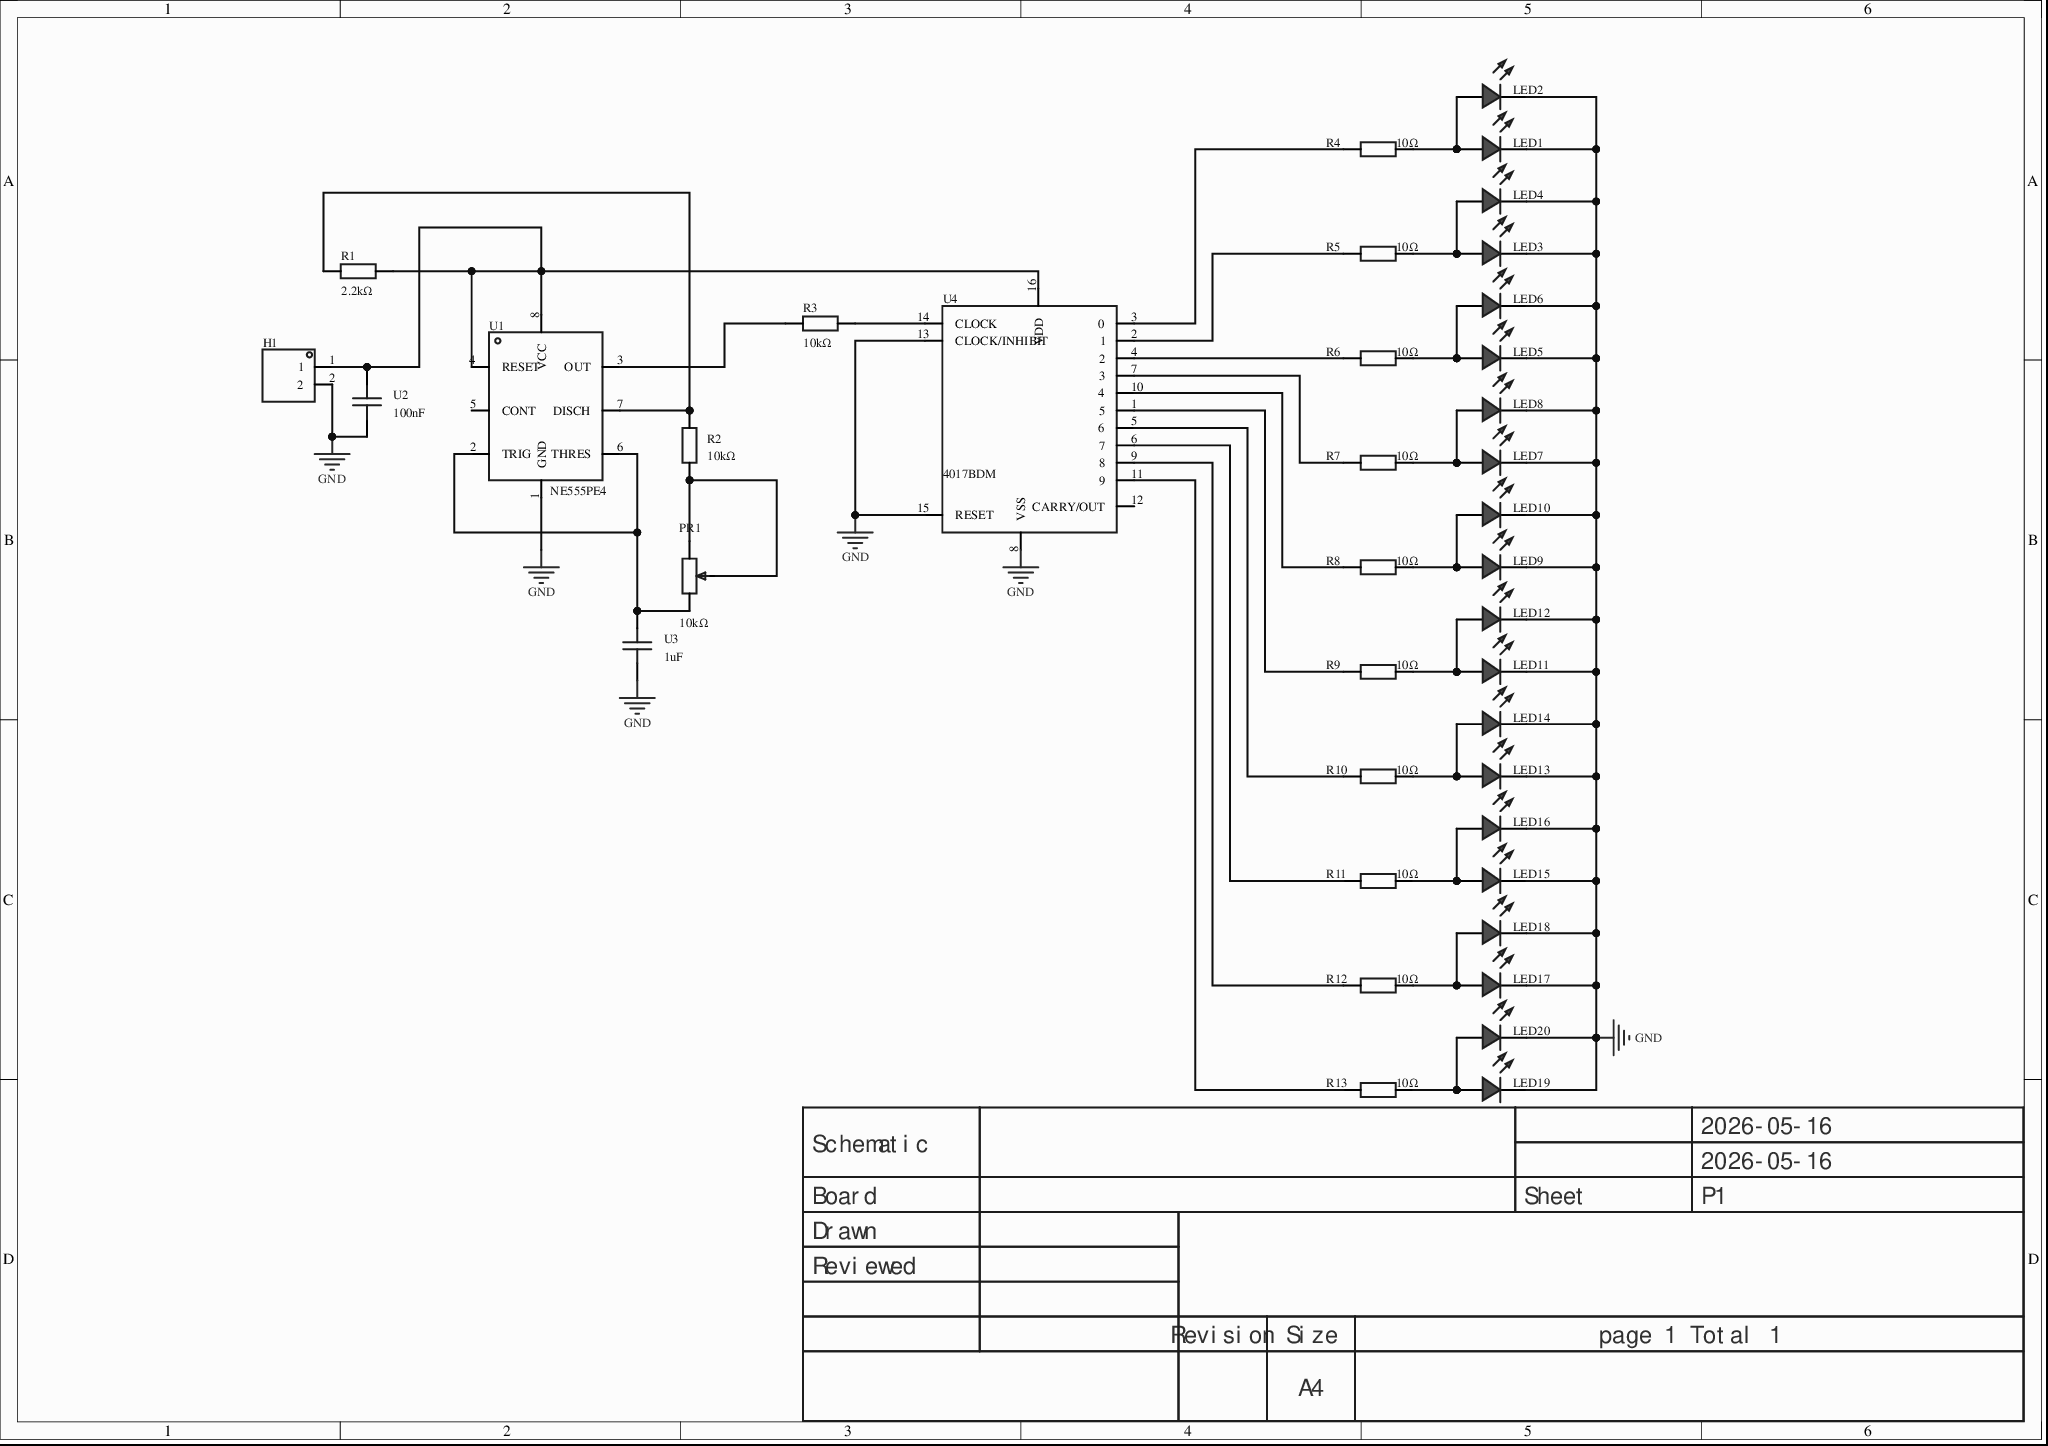
[diagram p0: MISC51889-3.schdoc]
# Altium project MISC51889-2.PrjPcb
1 sheet, 39 parts. Net scope: global (net labels, ports and power ports of the same name join across sheets).
Board file: MISC51889.pcbdoc

## Sheet MISC51889-3.schdoc
size 297 x 209 mm; Version: V1.0; @Project Name: MISC51889; @Update Date: 2026-05-16; @Create Date: 2026-05-16; @Board Name: MISC51889; @Create Time: 21:48:10; @Page Count: 1; @Page No: 1; @Schematic Name: MISC51889; @Update Time: 21:48:10; Size: A4

### Parts
H1  (no value)  [HDR-TH_2P-P2.54-V-M-1]
LED1  (no value)  [LED_TH-3mm]
LED2  (no value)  [LED_TH-3mm]
LED3  (no value)  [LED_TH-3mm]
LED4  (no value)  [LED_TH-3mm]
LED5  (no value)  [LED_TH-3mm]
LED6  (no value)  [LED_TH-3mm]
LED7  (no value)  [LED_TH-3mm]
LED8  (no value)  [LED_TH-3mm]
LED9  (no value)  [LED_TH-3mm]
LED10  (no value)  [LED_TH-3mm]
LED11  (no value)  [LED_TH-3mm]
LED12  (no value)  [LED_TH-3mm]
LED13  (no value)  [LED_TH-3mm]
LED14  (no value)  [LED_TH-3mm]
LED15  (no value)  [LED_TH-3mm]
LED16  (no value)  [LED_TH-3mm]
LED17  (no value)  [LED_TH-3mm]
LED18  (no value)  [LED_TH-3mm]
LED19  (no value)  [LED_TH-3mm]
LED20  (no value)  [LED_TH-3mm]
PR1  10kΩ  [R_3296]
R1  2.2kΩ  [Res_1/8W]
R2  10kΩ  [Res_1/8W]
R3  10kΩ  [Res_1/8W]
R4  10Ω  [Res_1/8W]
R5  10Ω  [Res_1/8W]
R6  10Ω  [Res_1/8W]
R7  10Ω  [Res_1/8W]
R8  10Ω  [Res_1/8W]
R9  10Ω  [Res_1/8W]
R10  10Ω  [Res_1/8W]
R11  10Ω  [Res_1/8W]
R12  10Ω  [Res_1/8W]
R13  10Ω  [Res_1/8W]
U1  NE555PE4  [PDIP-8_L9.6-W6.4-P2.54-LS7.9-BL-1]
U2  100nF  [CAP-TH_L5.0-W2.5-P5.00-D1.0]
U3  1uF  [CAP-TH_L5.0-W2.5-P5.00-D1.0]
U4  4017BDM  [PDIP-16_L19.3-W6.5-P2.54-LS7.6-BL]

### Nets
GND: H1.2 LED1.2(A) LED2.2(A) LED3.2(A) LED4.2(A) LED5.2(A) LED6.2(A) LED7.2(A) LED8.2(A) LED9.2(A) LED10.2(A) LED11.2(A) LED12.2(A) LED13.2(A) LED14.2(A) LED15.2(A) LED16.2(A) LED17.2(A) LED18.2(A) LED19.2(A) LED20.2(A) U1.1(GND) U2.2 U3.2 U4.8(VSS) U4.13(CLOCK/INHIBIT) U4.15(RESET)
NetH1_1: H1.1 R1.2 U1.4(RESET) U1.8(VCC) U2.1 U4.16(VDD)
NetLED1_1: LED1.1(C) LED2.1(C) R4.2
NetLED3_1: LED3.1(C) LED4.1(C) R5.2
NetLED5_1: LED5.1(C) LED6.1(C) R6.2
NetLED7_1: LED7.1(C) LED8.1(C) R7.2
NetLED9_1: LED9.1(C) LED10.1(C) R8.2
NetLED11_1: LED11.1(C) LED12.1(C) R9.2
NetLED13_1: LED13.1(C) LED14.1(C) R10.2
NetLED15_1: LED15.1(C) LED16.1(C) R11.2
NetLED17_1: LED17.1(C) LED18.1(C) R12.2
NetLED19_1: LED19.1(C) LED20.1(C) R13.2
NetPR1_1: PR1.1 U1.2(TRIG) U1.6(THRES) U3.1
NetPR1_2: PR1.2 PR1.3 R2.1
NetR1_1: R1.1 R2.2 U1.7(DISCH)
NetR3_1: R3.1 U1.3(OUT)
NetR3_2: R3.2 U4.14(CLOCK)
NetR4_1: R4.1 U4.3(0)
NetR5_1: R5.1 U4.2(1)
NetR6_1: R6.1 U4.4(2)
NetR7_1: R7.1 U4.7(3)
NetR8_1: R8.1 U4.10(4)
NetR9_1: R9.1 U4.1(5)
NetR10_1: R10.1 U4.5(6)
NetR11_1: R11.1 U4.6(7)
NetR12_1: R12.1 U4.9(8)
NetR13_1: R13.1 U4.11(9)

Not connected (* = marked no-connect by the designer): U1 5(CONT); U4 12(CARRY/OUT)

### Notes on the sheet
- 2026-05-16
- Schematic
- Board
- Sheet
- P1
- Drawn
- Reviewed
- Revision
- Size
- A4
- page 1 Total 1

### Library data of the parts
H1 = HDR-M_2.54_1x2P: Symbol: 210S-1*2P L=11.6MMGold-plated black; ConvertToPcb: yes; ModelId: 79b2e9f2d70a4d68a1b7098f27c6d4c50819f05c4eef4c71ace90d822a990e87; ModelName: HDR-M-2.54_1x2; ModelTransform: 200,100,0,0,0,0,0,0,-118.11; Device: HDR-M_2.54_1x2P; AddInBom: yes; SupplierPart: C124375; Supplier Footprint: 插件; FootprintName: HDR-TH_2P-P2.54-V-M-1
LED1-LED20 = LED_TH-R_3mm: ConvertToPcb: yes; ModelId: a497c992633541038a38947cdc58012f0819f05c4eef4c71ace90d822a990e87; ModelName: LED-TH-3mm_R; ModelTransform: 141.274,153.327,0,0,0,0,-5.984,0,-137.795; Symbol: LED_TH-R; Device: LED_TH-R_3mm; AddInBom: yes; FootprintName: LED_TH-3mm; Supplier Footprint: 插件
PR1 = R_3296: ConvertToPcb: yes; ModelId: b182808559bb43bda9e7de64b64134cb0819f05c4eef4c71ace90d822a990e87; ModelName: 3296W; ModelTransform: 373.98,188.96,590.49,180,0,0,0,0,-140; Symbol: R_3296; Device: R_3296; AddInBom: yes; Supplier Footprint: 直插; FootprintName: R_3296; Value: 10kΩ
R1-R13 = Res_AXIAL-1/8W: Symbol: Resistor; ConvertToPcb: yes; ModelId: b2b5ae7ae4c642178fe0039925c86a3f0819f05c4eef4c71ace90d822a990e87; ModelName: RES-TH_BD1.8-L3.2-P7.20-D0.4; ModelTransform: 282.86,66.88,253.09,0,0,0,0,0,-191; Device: Res_AXIAL-1/8W; AddInBom: yes; Supplier Footprint: 轴向引线; FootprintName: Res_1/8W
  R1: Value: 2.2kΩ
  R2 R3: Value: 10kΩ
  R4-R13: Value: 10Ω
U1 = NE555PE4: NE555 single timer; Manufacturer: TI(德州仪器); Symbol: NE555PE4_1; AddInBom: yes; ModelId: 1b8eaf096e7944deafe216467068c10e0819f05c4eef4c71ace90d822a990e87; ModelTransform: 377.952,318.897,0,0,0,0,0,0,-118.11; Device: NE555PE4; LCSC Part Name: NE555PE4; SupplierPart: C2859604; ManufacturerPart: NE555PE4; Supplier Footprint: PDIP-8; JLCPCB Part Class: Extended Part; Supplier: LCSC; ConvertToPcb: yes; FootprintName: PDIP-8_L9.6-W6.4-P2.54-LS7.9-BL-1; ModelName: PDIP-8_L9.6-W6.4-P2.54-LS7.9-BL-1
U2 U3 = 100nF: Symbol: 100NF_C9900015256; AddInBom: yes; ModelId: 08e3d7481fc7486bb1b263873f51e1e10819f05c4eef4c71ace90d822a990e87; ModelName: CAP-TH_BD5.0-W2.5-P5.08; ModelTransform: 224.652,98.425,0,0,0,0,-0.005,0,-137.795; Device: 100nF; LCSC Part Name: 100nF; SupplierPart: C9900015256; Supplier Footprint: CAP-TH_L5.0-W2.5-P5.00-D1.0; JLCPCB Part Class: Extended Part; Supplier: LCSC; ConvertToPcb: yes; FootprintName: CAP-TH_L5.0-W2.5-P5.00-D1.0
  U2: ManufacturerPart: 100nF
  U3: Manufacturer Part: 1uF
U4 = 4017BDM: Operating voltage: 3V~15V; Number of components: 1; Bits per component: 5; Trigger type: positive edge; negative edge;; Manufacturer: TI(德州仪器); Symbol: 4017BDM_1; AddInBom: yes; ModelId: fbf64f1066904807ba848675b6d2e65d0819f05c4eef4c71ace90d822a990e87; ModelName: PDIP-16_L19.3-W6.5-H5.1-P2.54-LS7.6-BL; ModelTransform: 787.4,311.8104,0,0,0,0,0,0,-118.11; Logic Type: Decade counter; Direction: Up counter; Number of Elements: 1; Number of Bits per Element: 5; Reset Style: Asynchronous; Timing mode: Synchronous; Device: 4017BDM; LCSC Part Name: 4017BDM; SupplierPart: C3828355; ManufacturerPart: 4017BDM; Supplier Footprint: -; JLCPCB Part Class: Extended Part; Datasheet: https://atta.szlcsc.com/upload/public/pdf/source/20230921/138E63DECC921583B49D9ECA49507D15.pdf; Supplier: LCSC; ConvertToPcb: yes; FootprintName: PDIP-16_L19.3-W6.5-P2.54-LS7.6-BL; Supply Voltage: 3V~15V; Trigger Type: Positive edge; negative edge; Operating Temperature: -40℃~+85℃